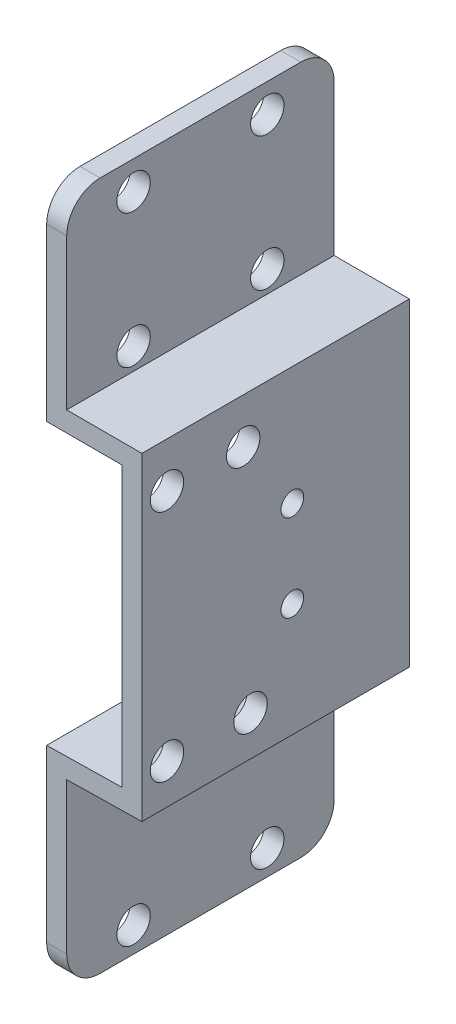
SolidWorks part; units mm, degrees
ref_plane "Front Plane" through (0, 0, 0) normal (0, 0, 1) x (1, 0, 0)
ref_plane "Top Plane" through (0, 0, 0) normal (0, 1, 0) x (1, 0, 0)
ref_plane "Right Plane" through (0, 0, 0) normal (1, 0, 0) x (0, 0, -1)
sketch "Sketch1" plane through (0, 0, 0) normal (0, 0, 1) x (1, 0, 0)
  line L0 (-5.625, 51.525) -> (-5.625, 20.975)
  line L2 (5.625, 20.975) -> (5.625, -20.7773)
  line L4 (-5.625, -20.9746) -> (-5.625, -51.525)
  line L5 (5.625, -20.7773) -> (-5.625, -20.9746)
  line L6 (-5.625, 20.975) -> (5.625, 20.975)
extrude "Extrude-Thin1" add sketch "Sketch1" along normal mid plane 40 thin contours L0 L6 L2 L5 thin type one direction reverse wall 3
fillet "Fillet1" radius 5 4 edges at (-4.125, -51.525, -20) (-4.125, -51.525, 20) (-4.125, 51.525, -20) (-4.125, 51.525, 20)
hole_wizard "Size mm Dowel Hole1" positions "Sketch2" profile "Sketch5" hole size "Ø5.0" standard "GB" end condition through all
sketch "Sketch2" plane through (8.625, 0, 0) normal (1, 0, 0) x (0, 0, -1)
  point P0 (-3.75, -17.7681)
  point P3 (-16.25, -17.7681)
  point P6 (-4.8581, 17.2319)
  point P9 (-16.25, 17.2319)
  point P12 (10, 47.2319)
  point P15 (10, 27.2319)
  point P18 (-10, 27.2319)
  point P21 (-10, 47.2319)
  point P24 (10, -47.7681)
  point P27 (10, -27.7681)
  point P30 (-10, -27.7681)
  point P33 (-10, -47.7681)
sketch "Sketch5" plane through (8.625, -17.7681, 3.75) normal (0, 1, 0) x (0, 0, -1)
  line L0 (0, 0) -> (0, 14.25)
  line L1 (0, 14.25) -> (2.5, 14.25)
  line L2 (2.5, 14.25) -> (2.5, 0)
  line L5 (2.5, 0) -> (0, 0)
  line L11 (0, -6.35) -> (0, 107.95) construction
  dimension "通孔孔直径" = 5
  dimension "通孔孔深度" = 14.25
hole_wizard "M4 Tapped Hole1" positions "Sketch6" profile "Sketch7" tap size "M4" standard "GB" end condition through all
sketch "Sketch6" plane through (8.625, 0, 0) normal (1, 0, 0) x (0, 0, -1)
  point P0 (2.5, -6.7681)
  point P3 (2.5, 6.2319)
sketch "Sketch7" plane through (8.625, -6.7681, -2.5) normal (0, 1, 0) x (0, 0, -1)
  line L0 (0, 0) -> (0, 14.25)
  line L1 (0, 14.25) -> (1.7, 14.25)
  line L2 (1.7, 14.25) -> (1.7, 0)
  line L5 (1.7, 0) -> (0, 0)
  line L11 (0, -6.35) -> (0, 107.95) construction
  dimension "通孔螺纹孔钻头直径" = 3.4
  dimension "通孔螺纹孔钻头深度" = 14.25
cosmetic thread "Cosmetic Thread1" parameters "D2"=4
cosmetic thread "Cosmetic Thread2" parameters "D2"=4
